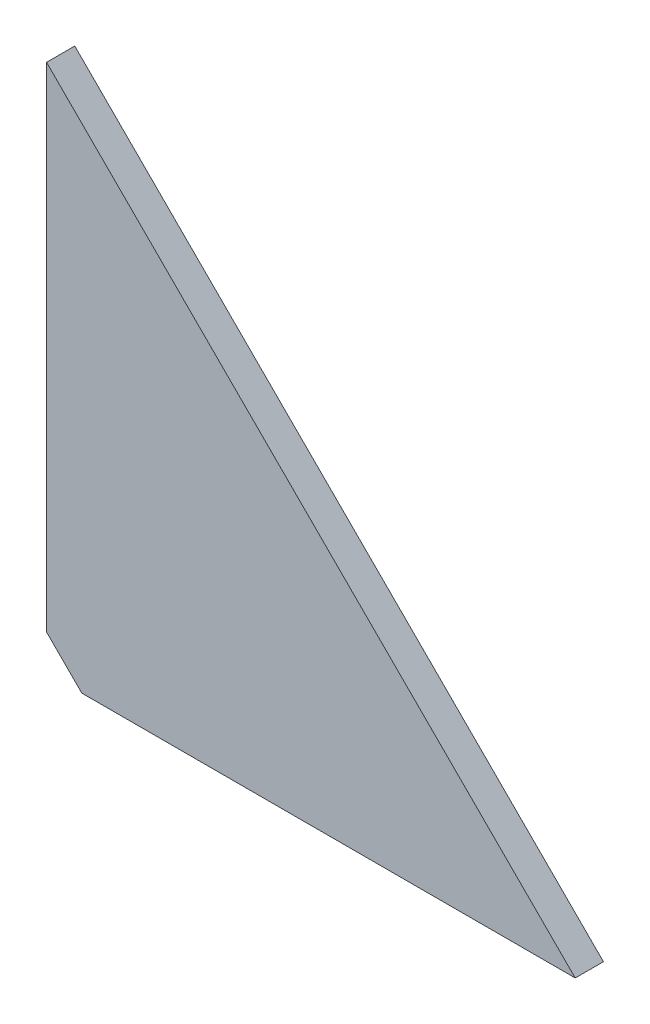
SolidWorks part; units mm, degrees
material "Q235B"
ref_plane "Front Plane" through (0, 0, 0) normal (0, 0, 1) x (1, 0, 0)
ref_plane "Top Plane" through (0, 0, 0) normal (0, 1, 0) x (1, 0, 0)
ref_plane "Right Plane" through (0, 0, 0) normal (1, 0, 0) x (0, 0, -1)
sketch "Sketch1" plane through (0, 0, 0) normal (0, 0, 1) x (1, 0, 0)
  line L0 (0, 0) -> (0, 300)
  line L1 (0, 300) -> (300, 0)
  line L2 (300, 0) -> (0, 0)
  dimension "D1" = 300
  dimension "D2" = 300
extrude "Boss-Extrude1" add sketch "Sketch1" along normal mid plane 16 contours L1 L2 L0
chamfer "Chamfer1" distance 20 angle 45 1 edges at (0, 0, 0)
